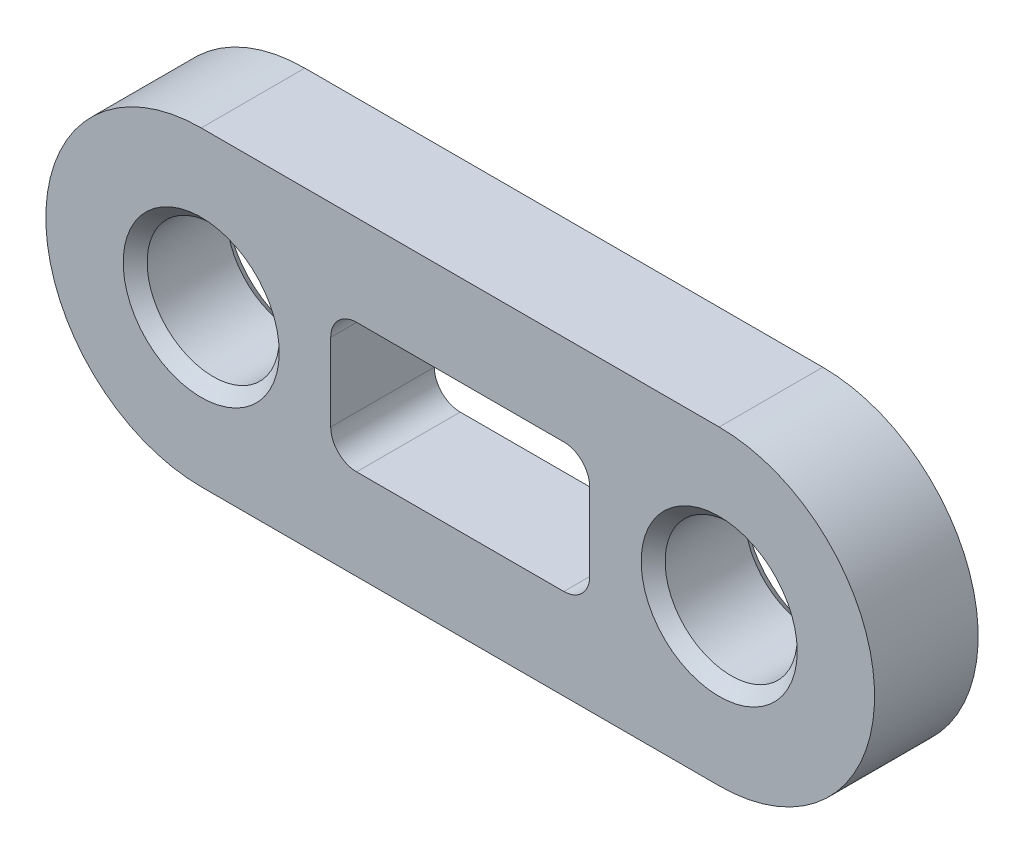
SolidWorks part; units mm, degrees
ref_plane "Front Plane" through (0, 0, 0) normal (0, 0, 1) x (1, 0, 0)
ref_plane "Top Plane" through (0, 0, 0) normal (0, 1, 0) x (1, 0, 0)
ref_plane "Right Plane" through (0, 0, 0) normal (1, 0, 0) x (0, 0, -1)
sketch "Sketch1" plane through (0, 0, 0) normal (0, 0, 1) x (1, 0, 0)
  line L0 (0, 12) -> (40, 12)
  line L1 (0, -12) -> (40, -12)
  line L3 (12, -5) -> (28, -5)
  line L4 (10, -3) -> (10, 3)
  line L5 (12, 5) -> (28, 5)
  line L6 (30, -3) -> (30, 3)
  line L7 (10, -5) -> (30, 5) construction
  line L8 (10, 5) -> (30, -5) construction
  arc A1 (0, 12) -> (0, -12) centre (0, 0) ccw
  arc A2 (40, -12) -> (40, 12) centre (40, 0) ccw
  arc A3 (28, 5) -> (30, 3) centre (28, 3) cw
  arc A4 (28, -5) -> (30, -3) centre (28, -3) ccw
  arc A5 (12, -5) -> (10, -3) centre (12, -3) cw
  arc A6 (10, 3) -> (12, 5) centre (12, 3) cw
  point P3 (20, 0)
  point P12 (20, -12)
  dimension "D1" = 24
  dimension "D5" = 2
  dimension "D2" = 40
  dimension "D3" = 20
  dimension "D4" = 10
extrude "Boss-Extrude1" add sketch "Sketch1" along normal mid plane 8
hole_wizard "M12 Tapped Hole1" positions "3DSketch1" profile "Sketch2" tap size "M12" standard "GB"
sketch3d "3DSketch1"
  line L0 (0, 0, 4) -> (0, 0, -4) construction
  point P0 (0, 0, 4)
sketch "Sketch2" plane through (0, 0, 4) normal (1, 0, 0) x (0, -1, 0)
  line L0 (0, 0) -> (0, 32.75)
  line L1 (0, 32.75) -> (5.1, 29.6856)
  line L2 (5.1, 29.6856) -> (5.1, 0.925)
  line L3 (5.1, 0.925) -> (6.025, 0)
  line L5 (6.025, 0) -> (0, 0)
  line L6 (-5.1, 0.925) -> (-6.025, 0) construction
  line L10 (0, 32.75) -> (-5.1, 29.6856) construction
  line L11 (0, -6.35) -> (0, 107.95) construction
  dimension "螺纹孔钻头直径" = 10.2
  dimension "螺纹孔钻头深度" = 32.75
  dimension "近端锥形沉头孔直径" = 12.05
  dimension "近端锥形沉头孔角度" = 90
  dimension "导头角度" = 118
cosmetic thread "Hole Thread1" parameters "D1"=24, "D2"=12
mirror "Mirror1" about plane through (0, 0, 0) normal (0, 0, 1) of "M12 Tapped Hole1"
ref_plane "Plane1" through (20, 0, 0) normal (1, 0, 0) x (0, 0, -1)
mirror "Mirror2" about plane through (20, 0, 0) normal (1, 0, 0) of "Mirror1", "M12 Tapped Hole1"
cosmetic thread "Hole Thread2"
